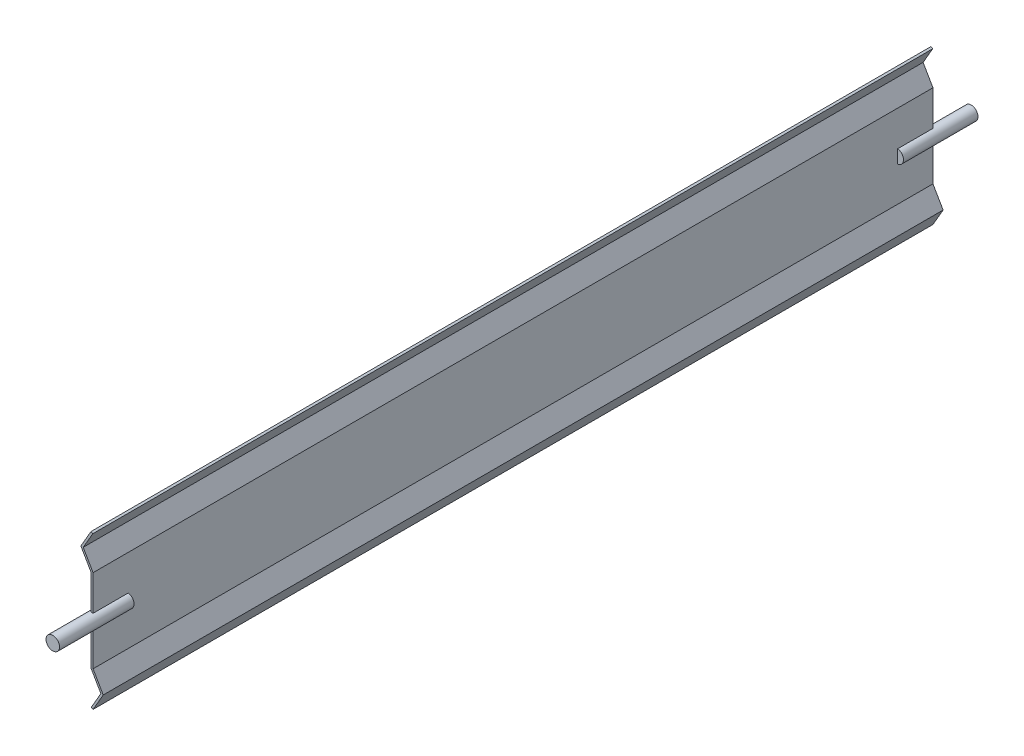
SolidWorks part; units mm, degrees
ref_plane "Front Plane" through (0, 0, 0) normal (0, 0, 1) x (1, 0, 0)
ref_plane "Top Plane" through (0, 0, 0) normal (0, 1, 0) x (1, 0, 0)
ref_plane "Right Plane" through (0, 0, 0) normal (1, 0, 0) x (0, 0, -1)
sketch "Sketch1" plane through (0, 0, 0) normal (0, 0, 1) x (1, 0, 0)
  line L0 (0, 0) -> (7.5, 12.9904)
  line L1 (7.5, 12.9904) -> (0, 25.9808)
  line L2 (0, 25.9808) -> (0, 87.4212)
  line L3 (0, 87.4212) -> (-7.2679, 100.0096)
  line L4 (-7.2679, 100.0096) -> (-0.201, 112.25)
  line L5 (-1.299, 0.75) -> (5.7679, 12.9904)
  line L6 (5.7679, 12.9904) -> (-1.5, 25.5788)
  line L7 (-1.5, 25.5788) -> (-1.5, 87.0192)
  line L8 (-1.5, 87.0192) -> (-9, 100.0096)
  line L9 (-9, 100.0096) -> (-1.5, 113)
  line L10 (-0.201, 112.25) -> (-1.5, 113)
  line L11 (0, 0) -> (-1.299, 0.75)
  dimension "D1" = 1.5
  dimension "D2" = 120
  dimension "D3" = 150
  dimension "D4" = 120
  dimension "D5" = 150
  dimension "D6" = 113
  dimension "D7" = 15
  dimension "D8" = 15
  dimension "D9" = 15
  dimension "D10" = 15
extrude "Boss-Extrude1" add sketch "Sketch1" along normal mid plane 620
sketch "Sketch2" plane through (0, 0, 310) normal (0, 0, 1) x (1, 0, 0)
  line L0 (-1.5, 56.5) -> (0, 56.5) construction
  line L1 (-1.5, 87.0192) -> (-1.5, 25.5788) construction
  line L2 (0, 25.9808) -> (0, 87.4212) construction
  circle A0 centre (-0.75, 56.5) radius 5
  dimension "D1" = 10
  dimension "D2" = 56.5
extrude "Boss-Extrude2" add sketch "Sketch2" along normal blind 29 and the other way blind 26
mirror "Mirror1" about plane through (0, 0, 0) normal (0, 0, 1) of "Boss-Extrude2"
